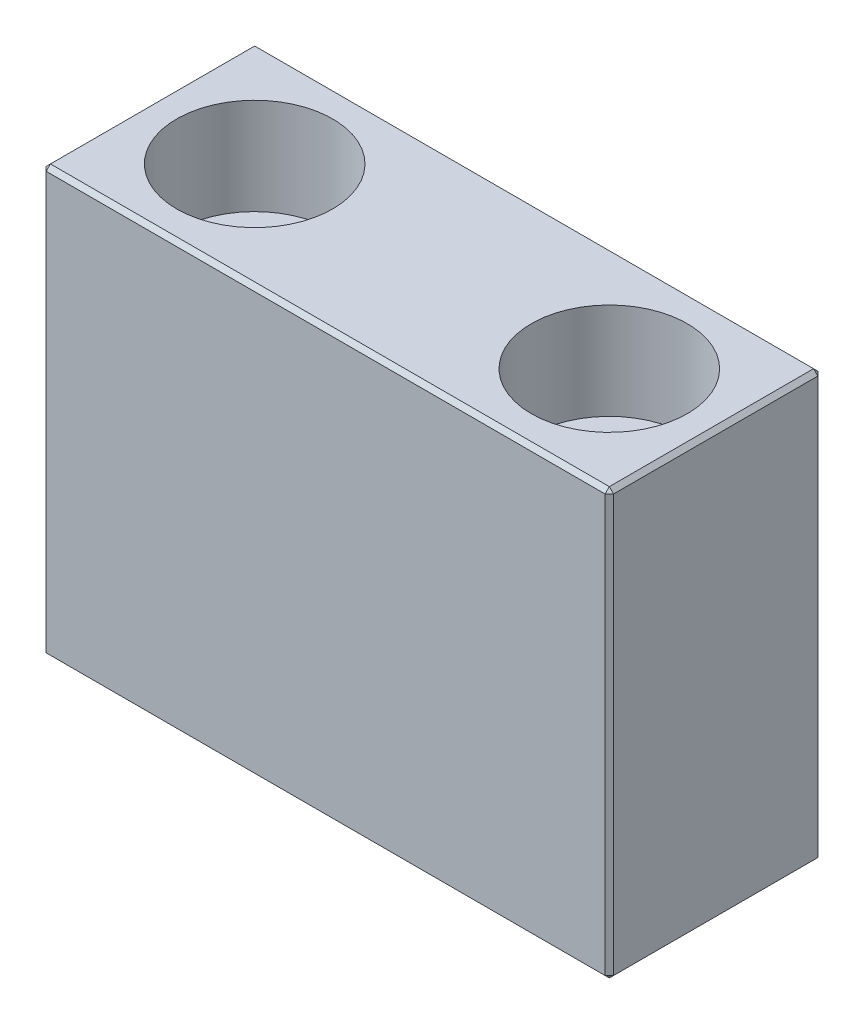
SolidWorks part; units mm, degrees
material "45号钢"
ref_plane "Front" through (0, 0, 0) normal (0, 0, 1) x (1, 0, 0)
ref_plane "Top" through (0, 0, 0) normal (0, 1, 0) x (1, 0, 0)
ref_plane "Right" through (0, 0, 0) normal (1, 0, 0) x (0, 0, -1)
sketch "草图1" plane through (0, 0, 0) normal (0, 0, 1) x (1, 0, 0)
  line L1 (-20, 15) -> (20, 15)
  line L2 (-20, 15) -> (-20, -15)
  line L3 (-20, -15) -> (20, -15)
  line L4 (20, 15) -> (20, -15)
  line L5 (-20, 15) -> (20, -15) construction
  line L6 (-20, -15) -> (20, 15) construction
  point P0 (0, 0)
  dimension "D1" = 40
  dimension "D2" = 30
extrude "凸台-拉伸1" add sketch "草图1" along normal blind 15
hole_wizard "打孔尺寸根据内六角圆柱头螺钉的类型1" positions "草图3" profile "草图2" counterbore size "M6" standard "Gb" end condition through all
sketch "草图3" plane through (0, 15, 0) normal (0, 1, 0) x (1, 0, 0)
  line L0 (20, -7.5) -> (12.5, -7.5) construction
  line L1 (20, -15) -> (20, 0) construction
  line L3 (0, 0) -> (0, -15) construction
  line L4 (20, -15) -> (-20, -15) construction
  point P0 (-12.5, -7.5)
  point P2 (12.5, -7.5)
  dimension "D1" = 25
sketch "草图2" plane through (-12.5, 15, 7.5) normal (1, 0, 0) x (0, 0, 1)
  line L0 (0, 0) -> (0, 30)
  line L1 (0, 30) -> (3.3, 30)
  line L3 (3.3, 30) -> (3.3, 6.8)
  line L4 (3.3, 6.8) -> (5.5, 6.8)
  line L5 (5.5, 6.8) -> (5.5, 0)
  line L7 (5.5, 0) -> (0, 0)
  line L11 (0, -6.35) -> (0, 107.95) construction
  dimension "通孔孔直径" = 6.6
  dimension "通孔孔深度" = 30
  dimension "柱形沉头孔直径" = 11
  dimension "柱形沉头孔深度" = 6.8
chamfer "倒角1" distance 0.3 angle 45 12 edges at (-20, 15, 7.5) (-20, -15, 7.5) (20, -15, 7.5) (0, -15, 15) (-20, 0, 15) (0, 15, 15) (20, 0, 15) (20, 15, 7.5) (0, 15, 0) (-20, 0, 0) (0, -15, 0) (20, 0, 0)
